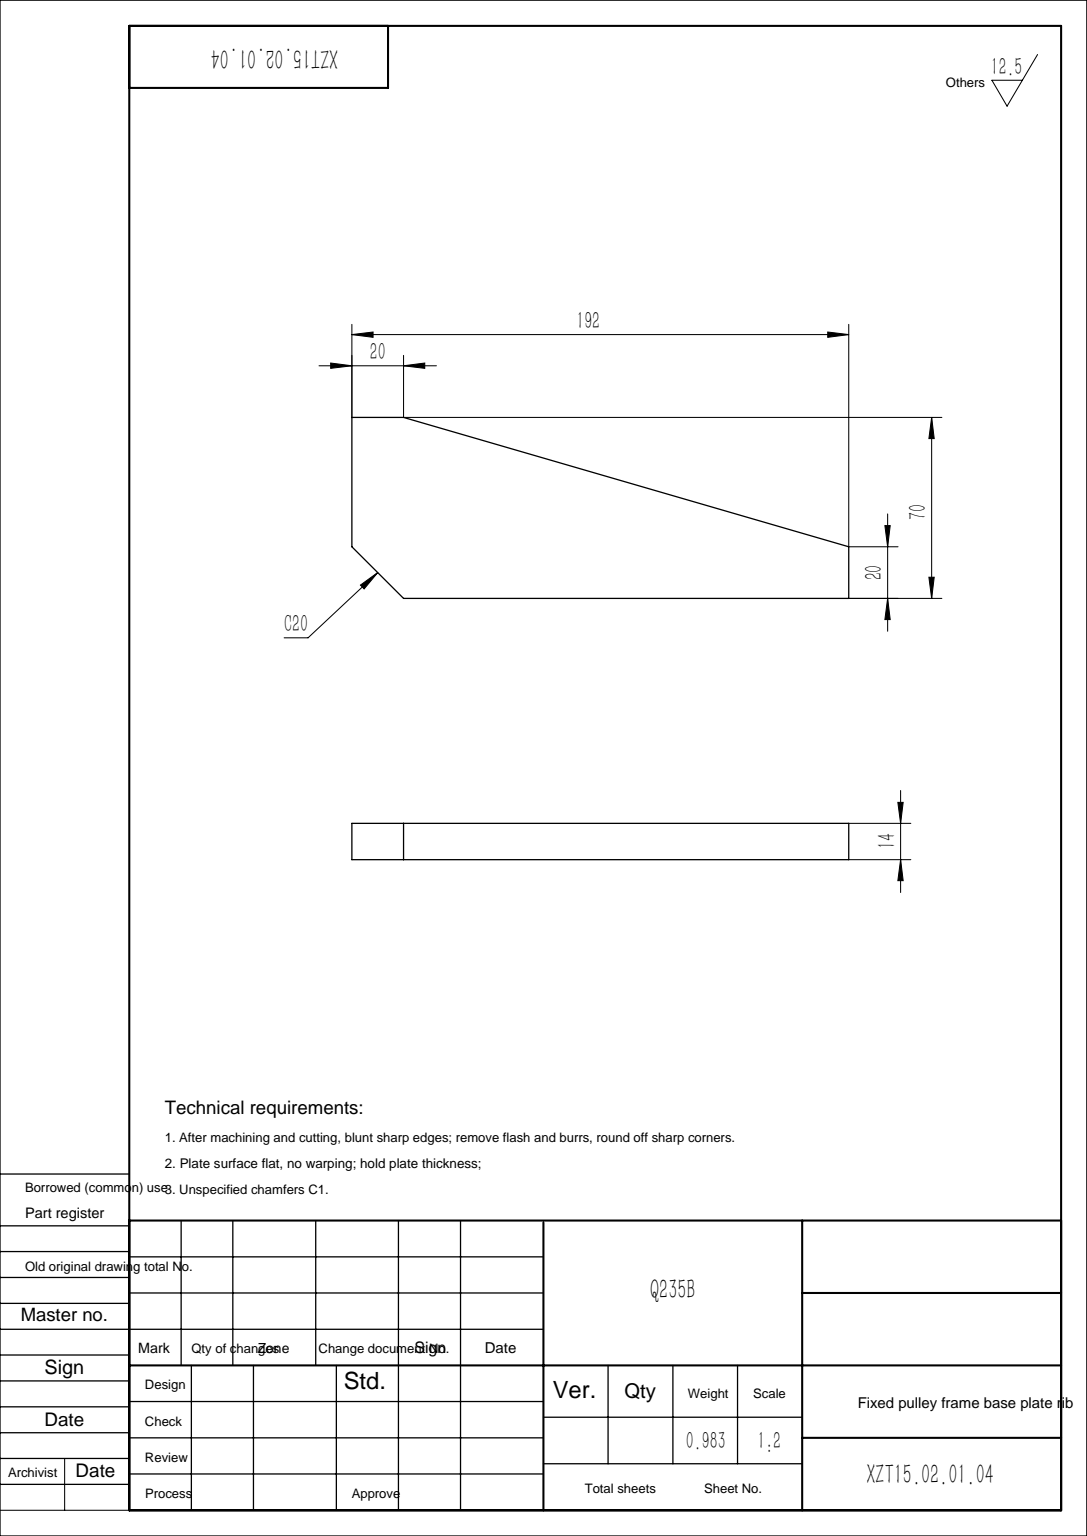
SolidWorks part; units mm, degrees
material "Q235B"
ref_plane "Front Plane" through (0, 0, 0) normal (0, 0, 1) x (1, 0, 0)
ref_plane "Top Plane" through (0, 0, 0) normal (0, 1, 0) x (1, 0, 0)
ref_plane "Right Plane" through (0, 0, 0) normal (1, 0, 0) x (0, 0, -1)
sketch "Sketch1" plane through (0, 0, 0) normal (0, 0, 1) x (1, 0, 0)
  line L0 (0, 0) -> (192, 0)
  line L1 (192, 0) -> (192, 20)
  line L2 (192, 20) -> (20, 70)
  line L3 (20, 70) -> (0, 70)
  line L4 (0, 70) -> (0, 0)
  dimension "D1" = 192
  dimension "D2" = 20
  dimension "D3" = 20
  dimension "D4" = 70
extrude "Boss-Extrude1" add sketch "Sketch1" along normal mid plane 14
chamfer "Chamfer1" distance 20 angle 45 1 edges at (0, 0, 0)
